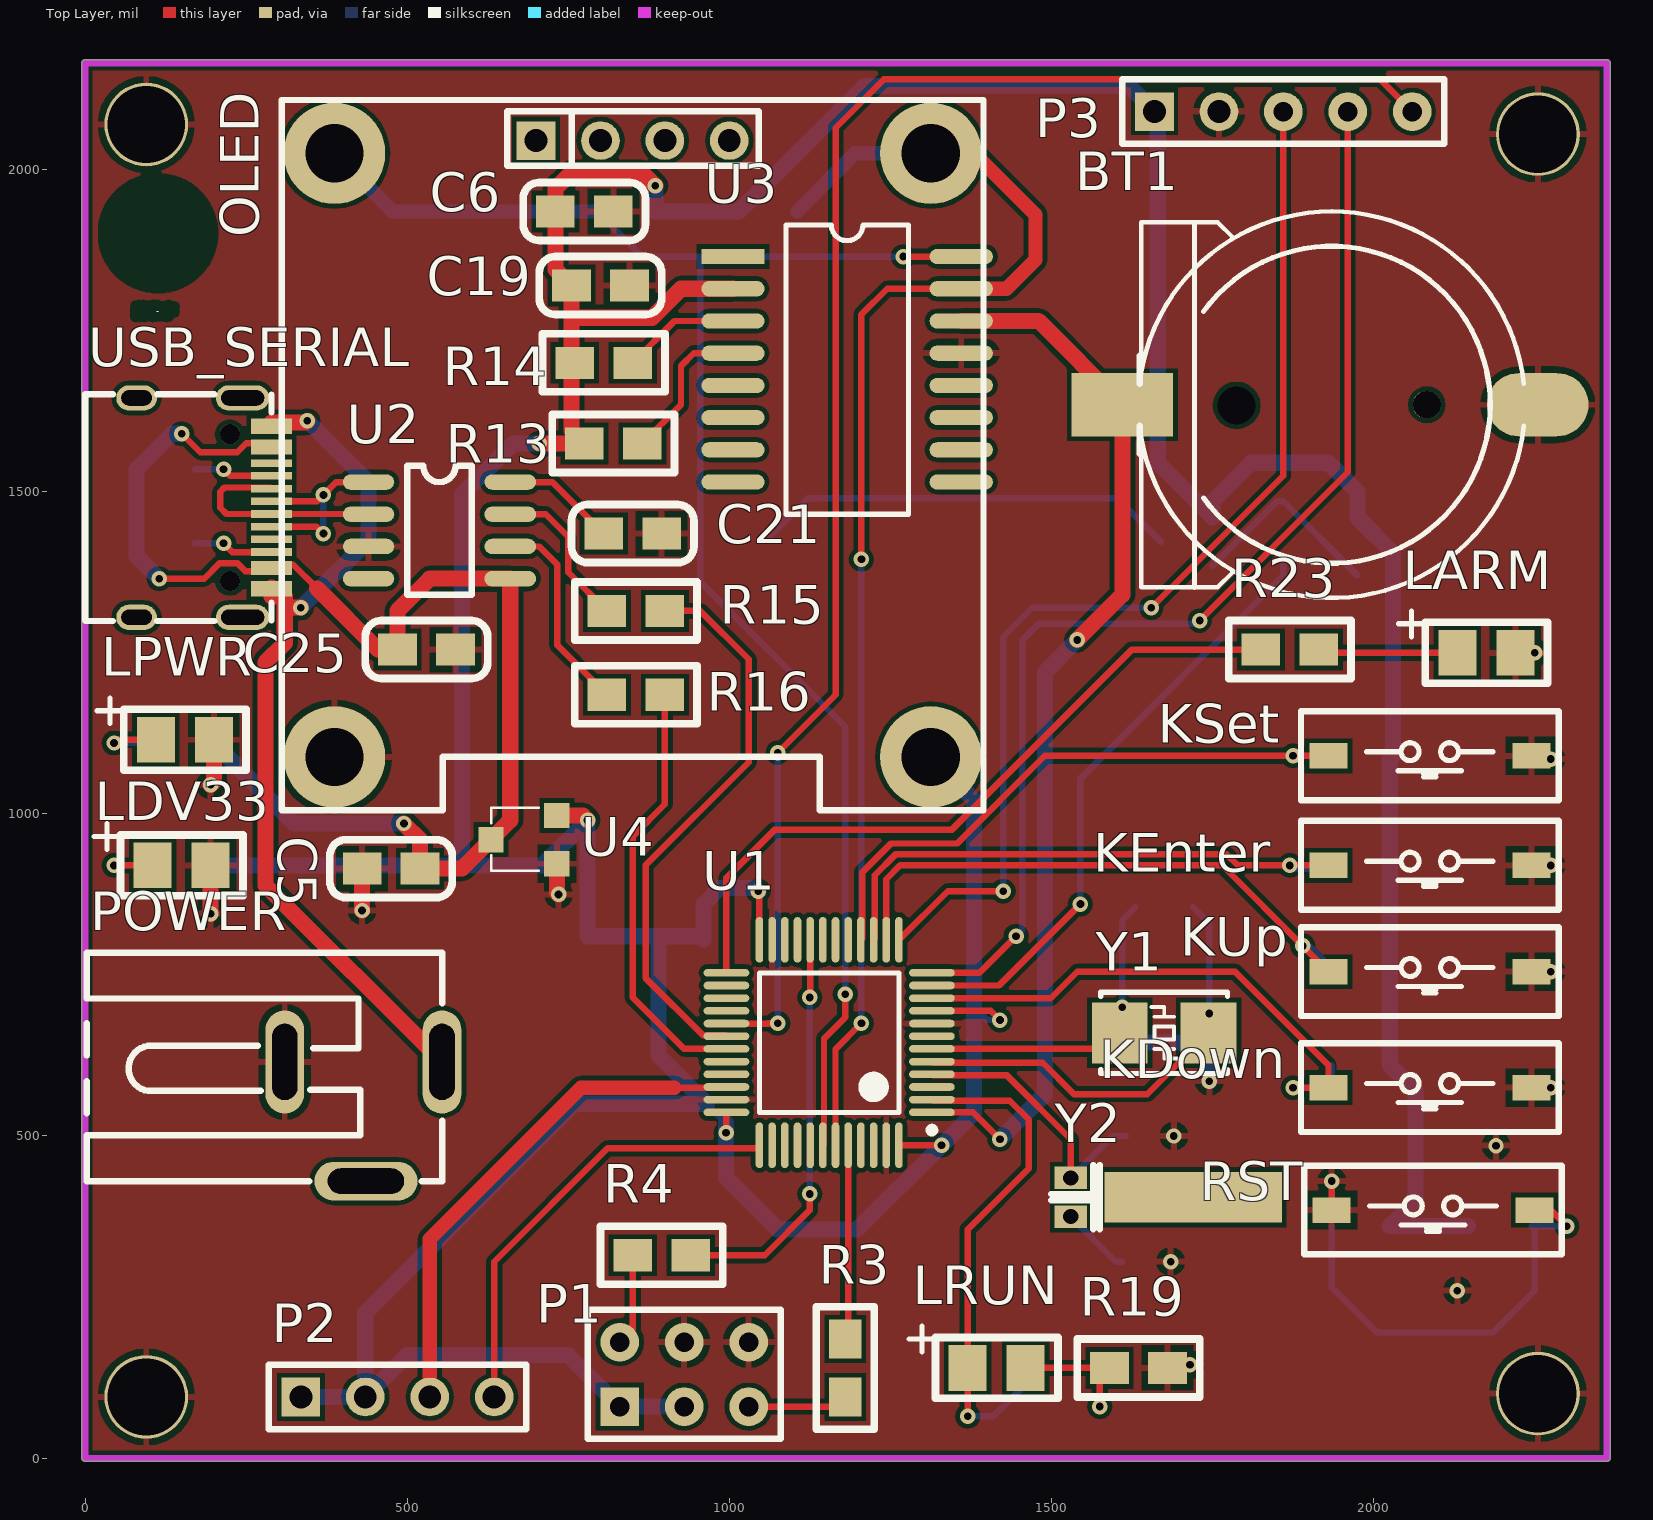
[diagram p0: Top Layer view]
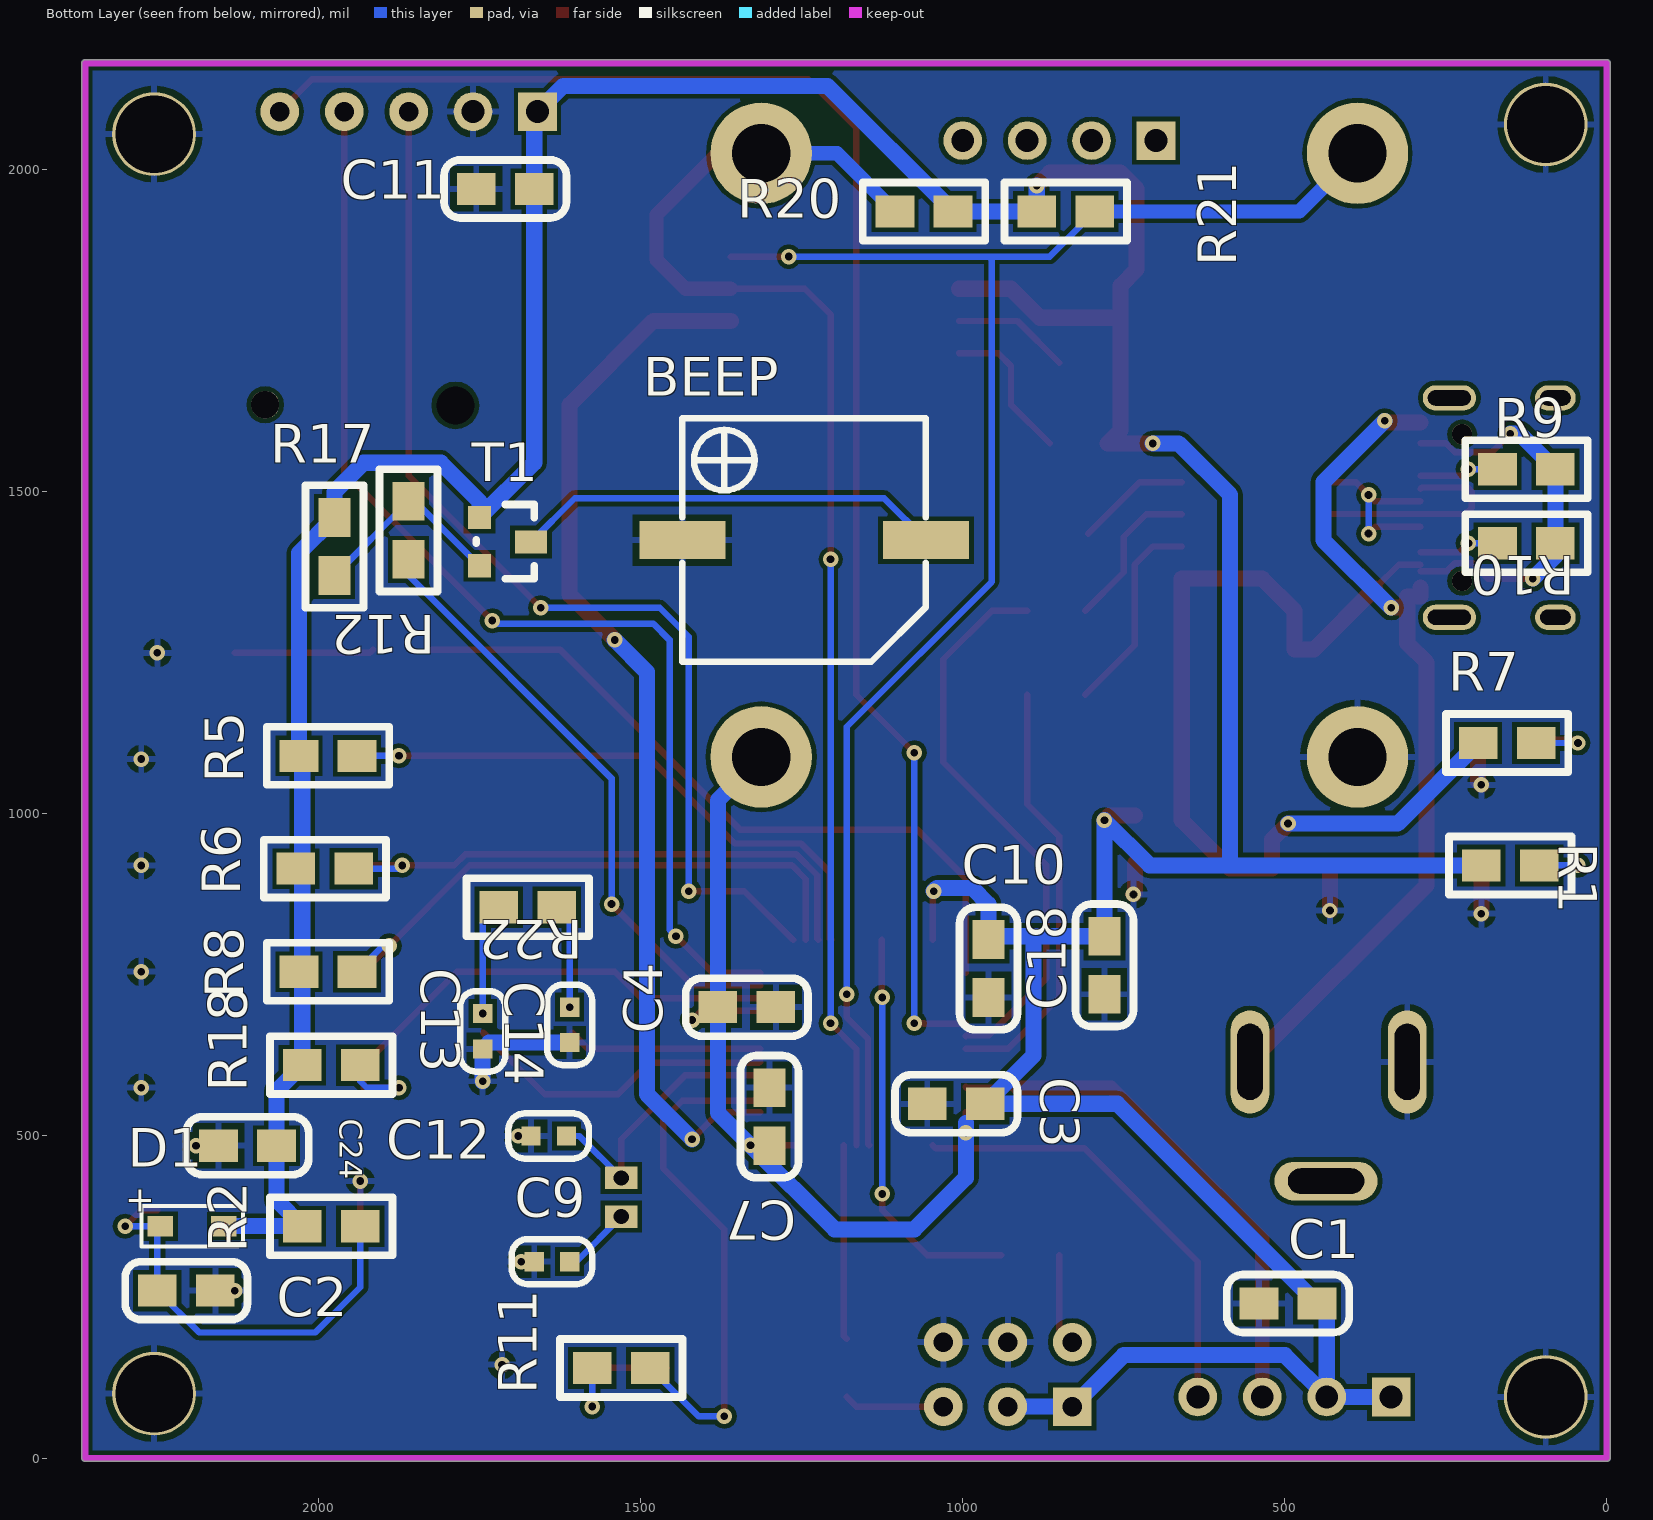
[diagram p1: Bottom Layer view, seen from below]
# Altium PCB MISC82121.PcbDoc
Units mil, origin at the board's own origin, x right, y up, seen from the top; angles counter-clockwise.
Board outline 2372.23 x 2175.38 mil, 2 copper layers (Top Layer, Bottom Layer); 66 components, 49 nets, 241 pads, 60 vias.

## Layer stack, top to bottom (the 12.6 mil dielectric is the usual default, probably not edited)
Top Solder: solder mask 0.4, Solder Resist, Dk 3.5
Top Layer: signal copper 1.4
Dielectric 1: dielectric 12.6, FR-4, Dk 4.8
Bottom Layer: signal copper 1.4
Bottom Solder: solder mask 0.4, Solder Resist, Dk 3.5

## Board outline
0,-5.01 cw(c0,0) -5.01,0 -5.01,2165.35 cw(c0,2165.35) 0,2170.37 2362.2,2170.37 cw(c2362.2,2165.35) 2367.22,2165.35 2367.22,0 cw(c2362.2,0) 2362.2,-5.01

## Design rules (kind name [scope] priority, off if disabled: settings)
Clearance [All] p1: gap=5 ignorepadtopadclearanceinfootprint=FALSE except(0: Arc-Text Track-Text SMDPad-Text THPad-Text Via-Text Fill-Text Poly-Text Region-Text Text-Text)
DiffPairsRouting [All] p1: maxlimit=10 minlimit=10 mostfreqgap=10 toplayer_minwidth=10 toplayer_maxwidth=15 toplayer_prefwidth=10 bottomlayer_minwidth=10 bottomlayer_maxwidth=15 bottomlayer_prefwidth=10 maxuncoupledlength=500
MinimumSolderMaskSliver [All] p1: minsoldermaskwidth=0
PolygonConnect [All] p1: connectstyle=Relief reliefconductorwidth=10 reliefentries=4 polygonreliefangle="90 Angle" airgapwidth=10
RoutingVias [All] p1: holewidth=28 width=50 viastyle="Through Hole" minholewidth=28 minwidth=50 maxholewidth=28 maxwidth=50
SilkToSilkClearance [All] p1: silktosilkclearance=0
SilkToSolderMaskClearance [IsPad] p1: minsilkscreentomaskgap=0 clearancetoexposedcopper=TRUE
SolderMaskExpansion [All] p1: expansion=4 istentingtop=FALSE
Width [All] p1: maxlimit=25 minlimit=10 preferedwidth=10
26 further rules are at their usual default settings.

## Classes and differential pairs
differential pair D: +D_P -D_N

## Components (designator, comment, footprint, x,y, rotation, side; value= is the part's Value field where it differs from the comment)
BEEP "Bell" HN9650B 1246.02,1425 r90 bottom
BT1 "1220_3V" CR1220 1935,1635 r180 top
C1 "104" C0805 450,240 r0 bottom
C2 "105" C0805 2160,260 r0 bottom
C3 "104" C0805 1055,550 r180 bottom
C4 "104" C0805 1290,700 r0 bottom
C5 "106" C0805 430,915 r0 top
C6 "106" C0805 820,1935 r180 top
C7 "104" C0805 1300,575 r270 bottom
C9 "10p" C0603 1665.11,305 r270 bottom
C10 "104" C0805 960,715 r90 bottom
C11 "106" C0805 1755,1970 r180 bottom
C12 "10p" C0603 1670.11,500 r270 bottom
C13 "22p" C0603 1745,634.89 r180 bottom
C14 "22p" C0603 1610,644.89 r180 bottom
C18 "105" C0805 780,810 r270 bottom net-tie
C19 "105" C0805 845,1820 r180 top
C21 "104" C0805 805,1435 r0 top
C24 "104" C0805 2155,485 r180 bottom
C25 "106" C0805 575,1255 r180 top net-tie
D1 "IN4148" D0805 2245,360 r180 bottom
KDown "SW-PB" KEY_8mm 2244.96,575 r180 top
KEnter "SW-PB" KEY_8mm 2244.96,920 r180 top
KSet "SW-PB" KEY_8mm 2244.96,1090 r180 top
KUp "SW-PB" KEY_8mm 2244.96,755 r180 top
LARM "RLED" LED0805 2130,1250 r0 top
LDV33 "RLED" LED0805 105,920 r0 top
LPWR "RLED" LED0805 110,1115 r0 top
LRUN "RLED" LED0805 1370,140 r0 top
OLED "OLED_IIC" OLED 305.51,1005.63 r0 top locked
P1 "IDC3*2" HDR2X3 830,80 r0 top
P2 "SWD" HDR1X4 335,95 r0 top
P3 "SIP5" HDR1X5 1660,2090 r0 top
POWER "5.2/2.1" SWC_SET 2.91,429.96 r0 top
R1 "Res2" R0805 195,920 r180 bottom
R2 "Res2" R0805 1935,360 r0 bottom
R3 "Res2" R0805 1180,185 r270 top
R4 "Res2" R0805 850,315 r0 top
R5 "Res2" R0805 1940,1090 r0 bottom
R6 "Res2" R0805 1945,915 r0 bottom
R7 "Res2" R0805 200,1110 r180 bottom
R8 "Res2" R0805 1940,755 r0 bottom
R9 "Res2" R0805 170,1535 r180 bottom
R10 "Res2" R0805 170,1420 r180 bottom
R11 "Res2" R0805 1575,140 r180 bottom
R12 "Res2" R0805 1860,1485 r270 bottom
R13 "Res2" R0805 865,1575 r180 top
R14 "Res2" R0805 850,1700 r180 top
R15 "Res2" R0805 810,1315 r0 top
R16 "Res2" R0805 810,1185 r0 top
R17 "Res2" R0805 1975,1370 r90 bottom
R18 "Res2" R0805 1935,610 r0 bottom
R19 "Res2" R0805 1680,140 r180 top
R20 "Res2" R0805 1105,1935 r180 bottom
R21 "Res2" R0805 795,1935 r0 bottom
R22 "Res2" R0805 1630,855 r0 bottom
R23 "Res2" R0805 1915,1255 r180 top
RST "SW-PB" KEY_8mm 2249.96,385 r180 top
T1 "S8550" SOT-23 1750,1460 r270 bottom
U1 "STM32F103C8T6A" LQFP48 1155,645 r180 top
U2 "CH340N" SO-8 440,1515 r0 top
U3 "DS3231SN" SOP-16 1005.67,1865 r0 top
U4 "XC6206P332MR" SOT-23S 732.36,922.6 r90 top
USB_SERIAL "type_C_16pins" TYPE_C_16PIN 289.45,1475.28 r90 top
Y1 "8MHZ" "OSC 5032-2P" 1675,660 r0 top
Y2 "32.768K" OSC_2*6 1530,375 r0 top

## Footprints (in the part's own frame and the unit in brackets; to place one, negate y for a bottom-side part, rotate by r counter-clockwise, add the part's x,y. Pads: shape width x height; smd on the part's side, far side on the other; paste and mask are expansions set on the pad)
C0603 [mil]
  rect 30x30 smd: 1(0,0.11) 2(0,55.11)
  silkscreen extent -35,-35 35,90
C0805 [mil]
  rect 60x50 smd: 1(0,0) 2(90,0)
  silkscreen extent -50,-45 140,45
CR1220 [mm]
  round 1.1 hole 1.1 unplated: 0(-3.75,0)
  round 1.3 hole 1.5 unplated: 0(3.75,0.025)
  rect 4x2.5 smd: 1(8.255,0)
  oval 4x2.5 smd: 2(-8.128,0)
  silkscreen extent -7.57,-7.62 7.57,7.62
D0805 [mm]
  rect 1x0.8 smd: A(-0.005,0) K(2.495,0)
  silkscreen extent -0.76,-0.8 3.24,0.8
HDR1X4 [mil]
  rect 60x60 hole 35.43: 1(0,0)
  round 60 hole 35.43: 1(100,0) 2(200,0) 3(300,0)
  silkscreen extent -50,-50 350,50
HDR1X5 [mil]
  rect 60x60 hole 35.43: 1(0,0)
  round 60 hole 35.43: 2(100,0)
  round 60 hole 30: 3(200,0) 4(300,0) 5(400,0)
  silkscreen extent -50,-50 450,50
HDR2X3 [mil]
  rect 60x60 hole 30: 1(0,0)
  round 60 hole 30: 2(100,0) 3(200,0) 4(0,100) 5(100,100) 6(200,100)
  silkscreen extent -50,-50 250,150
HN9650B [mm] "Beep"
  rect 1.5x3.4 smd: 1(0,4.8) 2(0,-4.8)
  silkscreen extent -4.8,-4.8 4.8,4.8
KEY_8mm [mm]
  rect 1.5x1 smd: 1(0,0) 2(8,0)
  silkscreen extent -1.07,-1.75 9.09,1.75
LED0805 [mm]
  rect 1.5x1.8 smd: A(0,0) K(2.286,0)
  silkscreen extent -2.31,-1.2 3.56,1.65
LQFP48 [mm]
  oval 1.8x0.3 smd: 1(-4.05,2.75) 2(-4.05,2.25) 3(-4.05,1.75) 4(-4.05,1.25) 5(-4.05,0.75) 6(-4.05,0.25) 7(-4.05,-0.25) 8(-4.05,-0.75) 9(-4.05,-1.25) 10(-4.05,-1.75) 11(-4.05,-2.25) 12(-4.05,-2.75) 25(4.05,-2.75) 26(4.05,-2.25) 27(4.05,-1.75) 28(4.05,-1.25) 29(4.05,-0.75) 30(4.05,-0.25) 31(4.05,0.25) 32(4.05,0.75) 33(4.05,1.25) 34(4.05,1.75) 35(4.05,2.25) 36(4.05,2.75)
  oval 0.3x1.8 smd: 13(-2.75,-4.05) 14(-2.25,-4.05) 15(-1.75,-4.05) 16(-1.25,-4.05) 17(-0.75,-4.05) 18(-0.25,-4.05) 19(0.25,-4.05) 20(0.75,-4.05) 21(1.25,-4.05) 22(1.75,-4.05) 23(2.25,-4.05) 24(2.75,-4.05) 37(2.75,4.05) 38(2.25,4.05) 39(1.75,4.05) 40(1.25,4.05) 41(0.75,4.05) 42(0.25,4.05) 43(-0.25,4.05) 44(-0.75,4.05) 45(-1.25,4.05) 46(-1.75,4.05) 47(-2.25,4.05) 48(-2.75,4.05)
  silkscreen extent -4.18,-2.75 2.75,3.57, body extent -3.5,-3.5 3.5,3.5, height 1.6
OLED [mm]
  round 4 hole 2.3: 1(2.075,2.1) 2(25.585,2.1) 3(2.075,25.9) 4(25.585,25.9)
  rect 1.524x1.524 hole 0.9: 17(10.02,26.4)
  round 1.524 hole 0.9: 18(12.56,26.4) 19(15.1,26.4) 20(17.64,26.4)
  silkscreen extent 0,0 27.66,28
"OSC 5032-2P" [mm] "5mm*3.2mm*0.8mm(³¤*¿í*¸ß)"
  rect 2.2x2.4 smd: 1(-1.75,0) 2(1.75,0)
  silkscreen extent -2.5,-1.6 2.5,1.6, body extent -2.5,-1.6 2.5,1.6, height 0.86
OSC_2*6 [mil]
  rect 275.59x78.74 smd: 0(190,30)
  rect 50x35 hole 23.62: 1(0,0) 2(0,60)
  silkscreen extent -30,-20 45,80
R0805 [mil]
  rect 60x50 smd: 1(0,0) 2(90,0)
  silkscreen extent -50,-45 140,45
SO-8 [mil]
  oval 80x24 smd: 1(0,0) 2(0,-50) 3(0,-100) 4(0,-150) 5(220,-150) 6(220,-100) 7(220,-50) 8(220,0)
  silkscreen extent 60,-175 160,25
SOP-16 [mm]
  rect 2.5x0.6 smd: 1(0,0)
  oval 2.5x0.6 smd: 2(0,-1.27) 3(0,-2.54) 4(0,-3.81) 5(0,-5.08) 6(0,-6.35) 7(0,-7.62) 8(0,-8.89) 9(9,-8.89) 10(9,-7.62) 11(9,-6.35) 12(9,-5.08) 13(9,-3.81) 14(9,-2.54) 15(9,-1.27) 16(9,0)
  silkscreen extent 2.08,-10.16 6.92,1.25
SOT-23 [mil]
  rect 36x36 smd: 1(0,0) 2(75,0)
  rect 36x50 smd: 3(38,80)
  silkscreen extent -20,-5 95,85
SOT-23S [mm]
  rect 1x1 smd: 1(0,0) 2(1.9,0) 3(0.95,2.6)
  silkscreen extent -0.27,0.72 2.2,2.59
SWC_SET [mm]
  oval 4.064x1.524 hole 1 slot 3 at 0 deg: 0(11,0)
  oval 1.524x4.064 hole 1 slot 3 at 90 deg: 1(7.8,4.7) 3(14,4.7)
  silkscreen extent 0,0 14,9
TYPE_C_16PIN [mm]
  oval 1x2.1 hole 0.6 slot 1.7 at 90 deg: 16(-4.325,1.14) 17(4.325,1.14)
  oval 1x1.6 hole 0.6 slot 1.2 at 90 deg: 18(-4.325,5.32) 19(4.325,5.32)
  rect 0.31x1.6 smd: A1(3.35,0) A4(2.54,0) A9(-2.5,0) A12(-3.35,0) B1(-3.05,0) B12(3.05,0)
  rect 0.3x1.6 smd: A5(1.25,0) A6(0.25,0) A7(-0.25,0) A8(-1.25,0) B4(-2.25,0) B5(-1.75,0) B6(-0.75,0) B7(0.75,0) B8(1.75,0) B9(2.25,0)
  silkscreen extent -4.47,0 4.47,7.35

## Part data
BEEP: "Electrical Bell"
BT1: library part Battery, "Multicell Battery"
C1 C2 C3 C4 C5 C6 C7 C9 C10 C11 C12 C13 C14 C18 C19 C21 C24 C25: library part Cap, "Capacitor"
D1: library part Diode, "Default Diode"
KDown KEnter KSet KUp RST: "Switch"
LARM LDV33 LPWR LRUN: library part LED0, "Typical INFRARED GaAs LED"
OLED: library part OLED_I2C_I2164
R1 R2 R3 R4 R5 R6 R7 R8 R9 R10 R11 R12 R13 R14 R15 R16 R17 R18 R19 R20 R21 R22 R23: "Resistor"
U1: library part STM32F103C8T6
Y1 Y2: library part XTAL, "Crystal Oscillator"

## Free pads (board coordinates)
  round 130 hole 120: 2(95,2070) 3(95,95) 4(2255,100) 5(2255,2055)

## Via types
v1: diameter 24, hole 12, Top Layer to Bottom Layer, 58 vias
v2: diameter 31.5, hole 31.5, Top Layer to Bottom Layer, 2 vias

## Nets (pads, with @x,y where several pads share a name; then routed paths per layer and width w, separated by ;. In a path a pad name is that pad's centre, name@x,y a point inside that pad or via, vN(x,y) a via of type N, cw(c..) or ccw(c..) an arc to the next point about the centre after c; other vN are vias at no path point)
ALARM: R23.2 U1.25 | length 1123.5
  Top Layer w10: U1.25 995.55,900.55 1070,975 1345,975 1625,1255 R23.2
BELLN: R12.2 U1.11 | length 948.4
  Top Layer w10: U1.11 1418.58,733.58 v1(1545,860)
  Bottom Layer w10: v1(1545,860) 1545,1055 1860,1370 R12.2
BOOT0: R3.1 U1.44 | length 302.4
  Top Layer w10: R3.1 1184.53,189.53 U1.44
BOOT1: R4.2 U1.20 | length 633.6
  Top Layer w10: R4.2 1055,315 1125,385 v1(1125,410) ; v1(1125,715) 1125.47,715.47 U1.20
  Bottom Layer w10: v1(1125,410) v1(1125,715)
CHRXD: R15.2 U1.30 | length 885.1
  Top Layer w10: R15.2 955,1315 1030,1240 1030,1080 870,920 870,745.23 958.61,656.62 993.77,656.62 U1.30
CHTXD: R16.2 U1.31 | length 669.3
  Top Layer w10: R16.2 900,1015 850,965 850,715 929.84,635.16 U1.31
D_N: U2.2 USB_SERIAL.A7 USB_SERIAL.B7 | length 342.1
  Top Layer w10: USB_SERIAL.B7 287.67,1506.58 216.58,1506.58 210,1500 210,1475 219.57,1465.43 USB_SERIAL.A7 439.57,1465.43 U2.2
D_P: U2.1 USB_SERIAL.A6 USB_SERIAL.B6 | length 307.9
  Top Layer w10: USB_SERIAL.B6 359.25,1445.75 v1(370,1435) ; USB_SERIAL.A6 360.12,1485.12 v1(370,1495) 390,1515 U2.1
  Bottom Layer w10: v1(370,1435) v1(370,1495)
DS_INT: U1.17
DS_RST: R13.1 U3.4 | length 233.8
  Top Layer w10: R13.1 925,1635 925,1695 945,1715 U3.4
DV5V: C5.2 C25.2 R7.1 R9.2 R10.2 U2.5 U4.3 USB_SERIAL.A4 USB_SERIAL.A9 USB_SERIAL.B4 USB_SERIAL.B9 | length 2103
  Top Layer w10: v1(115,1365) 185,1365 209.24,1389.24 236.38,1389.24 248.77,1376.85 USB_SERIAL.A9 ; v1(150,1590) 178.69,1561.31 236.38,1561.31 250.34,1575.28 USB_SERIAL.A4 ; USB_SERIAL.B4 323.31,1386.69 360,1350
  Top Layer w25: 360,1350 455,1255 C25.2 485,1315 535,1365 U2.5 660,990 U4.3 585,915 C5.2 520,960 v1(495,985)
  Bottom Layer w25: v1(115,1365) 80,1400 R10.2 R9.2 135,1590 v1(150,1590) ; R7.1 325,985 v1(495,985)
DV33: C1.1 C3.2 C4.2 C6.2 C7.2 C10.2 C11.2 C18.1 C19.2 C24.2 D1.K OLED.2 P1.1 P1.2 P2.1 P3.1 R1.1 R2.2 R5.2 R6.2 R8.2 R13.2 R14.2 R17.2 R18.2 R20.2 R21.2 T1.1 U1.9 U1.24 U1.36 U1.48 U3.2 U4.2 | length 9305.2
  Top Layer w10: v1(995,505) 995,536.18 U1.36 ; v1(1045,880) 1046.73,878.27 U1.24 ; U1.48 v1(1329.45,485.55) v1@1330,485 ; U1.9 1405.79,694.21 v1(1420,680)
  Top Layer w25: v1(705,1575) R13.2 755,1595 755,1770 ; U4.2 772.6,997.4 v1(780,990) ; v1(885,1975) 865,1995 755,1995 730,1970 C6.2 730,1845 C19.2 755,1770 ; U3.2 925,1815 880,1770 755,1770
  Bottom Layer w10: C3.2 995,520 ; C4.2 1400,680 v1(1420,680)
  Bottom Layer w25: R1.1 585,920 ; P2.1@335,95 P2.1@435,95 ; v1(705,1575) 665,1575 585,1495 585,920 ; v1(885,1975) R21.2 R20.2 1210,2130 1620,2130 P3.1 1665,2085 C11.2 1665,1545 T1.1 1750,1485 1810,1545 1930,1545 1975,1500 R17.2 2030,1405 R5.2 2025,1085 R18.2 2065,570 C24.2 2065,400 R2.2 D1.K ; P1.2 P1.1 750,160 500,160 P2.1@435,95 ; 995,520 v1(995,505) 995,435 1075,355 1198.9,355 v1(1329.45,485.55) 1380,536.1 C4.2 1380,1021.1 OLED.2 ; v1(1045,880) 1040,885 985,885 960,860 C10.2 955,810 885,810 ; P2.1@435,95 435,225 C1.1 760,550 C3.2 890,625 890,805 885,810 ; 585,920 710,920 v1(780,990) C18.1 885,810
GND: BEEP.1 BT1.2 C1.2 C2.1 C3.1 C4.1 C5.1 C6.1 C7.1 C9.1 C10.1 C11.1 C12.1 C13.1 C14.1 C18.2 C19.1 C21.2 C24.1 C25.1 KDown.1 KEnter.1 KSet.1 KUp.1 LARM.K LDV33.K LPWR.K OLED.1 P1.5 P1.6 P3.2 pad.2 pad.3 pad.4 pad.5 POWER.1 R19.1 RST.2 U1.8 U1.23 U1.35 U1.47 U2.3 U3.13 U4.1 | length 494.9
  Top Layer w10: RST.2 v1(1935,430)
  Top Layer w25: v1(195,845) LDV33.K ; v1(195,1045) 200,1050 LPWR.K ; v1(430,850) C5.1 ; U4.1 732.36,877.64 v1(735,875)
  Bottom Layer w25: C14.1 1735,645 C13.1 v1(1745,585)
  other v1: 1715,145 2130,260 1685,305 2190,485 1690,500 2275,575 2275,755 2275,920 2275,1085 2250,1250
GNDU: POWER.3 USB_SERIAL.A1 USB_SERIAL.A12 USB_SERIAL.B1 USB_SERIAL.B12 | length 1337.3
  Top Layer w25: USB_SERIAL.B1@289.45,1351.25 USB_SERIAL.A12 289.45,1337.19 310,1337.19 310,1320 ; USB_SERIAL.A1 342.17,1607.17 v1(345,1610) ; v1(335,1320) 310,1320 ; POWER.3 280,889.09 280,1235 310,1265 310,1320
  Bottom Layer w25: v1(335,1320) 440,1425 440,1515 v1(345,1610)
KEYDOWN: KDown.2 R18.1 U1.10 | length 871.8
  Top Layer w10: U1.10 1498.9,713.9 1540,755 1785,755 1930,610 KDown.2 v1(1875,575)
  Bottom Layer w10: v1(1875,575) 1925,575 1935,585 R18.1
KEYENTER: KEnter.2 R6.1 U1.15 | length 902.8
  Top Layer w10: U1.15 1225.68,806.23 1225.68,904.72 1257.96,937 1772.04,937 1789.04,920 v1(1870,920) KEnter.2
  Bottom Layer w10: v1(1870,920) 1875,915 R6.1
KEYSET: KSet.2 R5.1 U1.16 | length 969.3
  Top Layer w10: U1.16 1205.99,806.23 1205.99,909.08 1250.92,954 1353.76,954 1489.76,1090 v1(1875,1090) KSet.2
  Bottom Layer w10: v1(1875,1090) R5.1
KEYUP: KUp.2 R8.1 U1.14 | length 924.3
  Top Layer w10: U1.14 1243.58,898.58 1265,920 1765,920 v1(1890,795) KUp.2
  Bottom Layer w10: v1(1890,795) 1900,795 R8.1
LED: LRUN.A R11.2 U1.2 | length 809
  Top Layer w10: U1.2 1316.23,554.64 1435.36,554.64 1465,525 1465,450 1370,355 LRUN.A v1(1370,65)
  Bottom Layer w10: v1(1370,65) 1410,65 R11.2
NetBEEP_2: BEEP.2 T1.3 | length 668
  Bottom Layer w10: BEEP.2 1122.05,1490 1602,1490 T1.3
NetC9_2: C9.2 Y2.1 | length 109
  Bottom Layer w10: Y2.1 1600,305 C9.2
NetC21_1: C21.1 U2.8 | length 178.1
  Top Layer w10: U2.8 725,1515 C21.1
NetLARM_1: LARM.A R23.1 | length 217.1
  Top Layer w10: R23.1 1920,1250 LARM.A
NetLDV33_1: LDV33.A R1.2 | length 120
  Top Layer w10: v1(45,920) LDV33.A
  Bottom Layer w10: v1(45,920) R1.2
NetLPWR_1: LPWR.A R7.2 | length 132.1
  Top Layer w10: v1(45,1110) 50,1115 LPWR.A
  Bottom Layer w10: v1(45,1110) R7.2
NetLRUN_2: LRUN.K R11.1 R19.2 | length 256.2
  Top Layer w10: LRUN.K R19.2 1575,125 v1(1575,80)
  Bottom Layer w10: v1(1575,80) R11.1
NetP1_3: P1.3 R3.2 | length 156.2
  Top Layer w10: P1.3 1165,80 R3.2
NetP1_4: P1.4 R4.1 | length 143.3
  Top Layer w10: P1.4 850,200 R4.1
NetR9_1: R9.1 USB_SERIAL.A5 | length 123.8
  Top Layer w10: v1(215,1535) 225.51,1524.49 USB_SERIAL.A5
  Bottom Layer w10: R9.1 v1(215,1535)
NetR10_1: R10.1 USB_SERIAL.B5 | length 125.1
  Top Layer w10: v1(215,1420) 228.62,1406.38 USB_SERIAL.B5
  Bottom Layer w10: R10.1 v1(215,1420)
NetR12_1: R12.1 R17.1 T1.2 | length 314.1
  Bottom Layer w10: T1.2 1850,1485 R12.1 R17.1
NetR14_1: R14.1 U3.3 | length 182.6
  Top Layer w10: R14.1 915,1765 U3.3
NetR15_1: R15.1 U2.7 | length 244.4
  Top Layer w10: U2.7 715,1465 750,1430 750,1375 R15.1
NetR16_1: R16.1 U2.6 | length 318.5
  Top Layer w10: U2.6 705,1415 733,1387 733,1262 R16.1
OSCIN: C13.2 R22.2 U1.5 Y1.2 | length 665.1
  Top Layer w10: U1.5 1316.23,613.69 1486.31,613.69 1535,565 1648.9,565 Y1.2
  Bottom Layer w10: R22.2 1745,830 v1(1745,690)
OSCOUT: C14.2 R22.1 U1.6 Y1.1 | length 465.2
  Top Layer w10: U1.6 1581.26,635.16 Y1.1
  Bottom Layer w10: v1(1610,700) 1610,835 R22.1
PPS: P3.5 U1.29 | length 2453.7
  Top Layer w10: U1.29 1059.53,674.53 1060,675 v1(1075,675) ; v1(1075,1095) 1165,1185 1165,2065 1240,2140 2010,2140 P3.5
  Bottom Layer w10: v1(1075,675) v1(1075,1095)
RESET: C2.2 D1.A R2.1 RST.1 | length 683.1
  Top Layer w10: RST.1 2275,385 v1(2300,360)
  Bottom Layer w10: R2.1 1935,265 2005,195 2185,195 C2.2 2250,355.21 D1.A v1(2300,360)
RTC_OSC1: U1.3
RTC_OSC2: C12.2 U1.4 Y2.2 | length 429.2
  Top Layer w10: U1.4 1316.23,594.01 1430.99,594.01 1530,495 Y2.2
  Bottom Layer w10: Y2.2 1595,500 C12.2
RXD2: P3.3 U1.13 | length 1691.6
  Top Layer w10: U1.13 1338.82,880 v1(1425,880) ; v1(1655,1320) 1860,1525 P3.3
  Bottom Layer w10: v1(1425,880) 1425,1275 1470,1320 v1(1655,1320)
SCL: OLED.3 R21.1 U1.42 U3.16 | length 2528.3
  Top Layer w10: U1.42 1146.94,487.33 1146.94,650.98 1180,684.04 v1(1180,720) ; v1(1270,1865) U3.16
  Bottom Layer w10: R21.1 865,1865 960,1865 ; v1(1180,720) 1180,1135 955,1360 955,1860 960,1865 ; v1(1270,1865) 960,1865
  Bottom Layer w22: OLED.3 477.52,1935 R21.1
SDA: OLED.4 R20.1 U1.43 U3.15 | length 2128.2
  Top Layer w10: U1.43 1164.84,634.84 v1(1205,675) ; v1(1205,1395) 1205,1775 1245,1815 U3.15
  Top Layer w22: OLED.4 1379.69,2025.31 1475,1930 1475,1860 1430,1815 U3.15
  Bottom Layer w10: v1(1205,675) v1(1205,1395)
  Bottom Layer w22: R20.1 1195.31,2025.31 OLED.4
SWDCLK: P2.3 U1.37 | length 696.5
  Top Layer w10: P2.3 635,305 811,481 1042.18,481 U1.37
SWDIO: P2.2 U1.34 | length 803.3
  Top Layer w10: 915,575 994.45,575 U1.34
  Top Layer w22: P2.2 535,340 770,575 915,575
TXD2: P3.4 U1.12 | length 1790.9
  Top Layer w10: U1.12 1388.27,753.27 v1(1445,810) ; v1(1730,1300) 1960,1530 P3.4
  Bottom Layer w10: v1(1445,810) 1455,820 1455,1270 1480,1295 1725,1295 v1(1730,1300)
USB_D+: U1.33
USB_D-: U1.32
VBAT: BT1.1 U1.1 U3.14 | length 1645.4
  Top Layer w10: U1.1 1378.27,536.73 v1(1420,495)
  Top Layer w25: U3.14 1480,1765 BT1.1 1610,1340 v1(1540,1270)
  Bottom Layer w25: v1(1420,495) 1490,565 1490,1220 v1(1540,1270)
pads on no net: BT1.0 OLED.17 OLED.18 OLED.19 OLED.20 POWER.0 U1.7 U1.18 U1.19 U1.21 U1.22 U1.26 U1.27 U1.28 U1.38 U1.39 U1.40 U1.41 U1.45 U1.46 U2.4 U3.1 U3.5 U3.6 U3.7 U3.8 U3.9 U3.10 U3.11 U3.12 USB_SERIAL.16 USB_SERIAL.17 USB_SERIAL.18 USB_SERIAL.19 USB_SERIAL.A8 USB_SERIAL.B8 Y2.0
copper on no net:
  other v2: 224.88,1361.5 224.88,1589.06

## Polygon pours and split planes (outlines as drawn)
GND on Bottom Layer "G" (solid, remove dead copper, pour order 8): -270,2325 -245,2350 2720,2350 2720,-90 2575,-235 2400,-60 -335,-60
GND on Top Layer "G" (solid, remove dead copper, pour order 6): -420,2390 3140,2390 3180,2350 2640,1810 2640,-330 -500,-330 -525,-305

## Keep-outs
Keep-Out Layer:
  lines w10: 2300,2165.35 2362.2,2165.35 2362.2,2143.25 2362.2,0 0,0 0,2165.35 2307.57,2165.35

## Silkscreen, mask and mechanical layers (free items; w line width, h text height)
Top Overlay:
  lines w1: 111,1780 114,1780